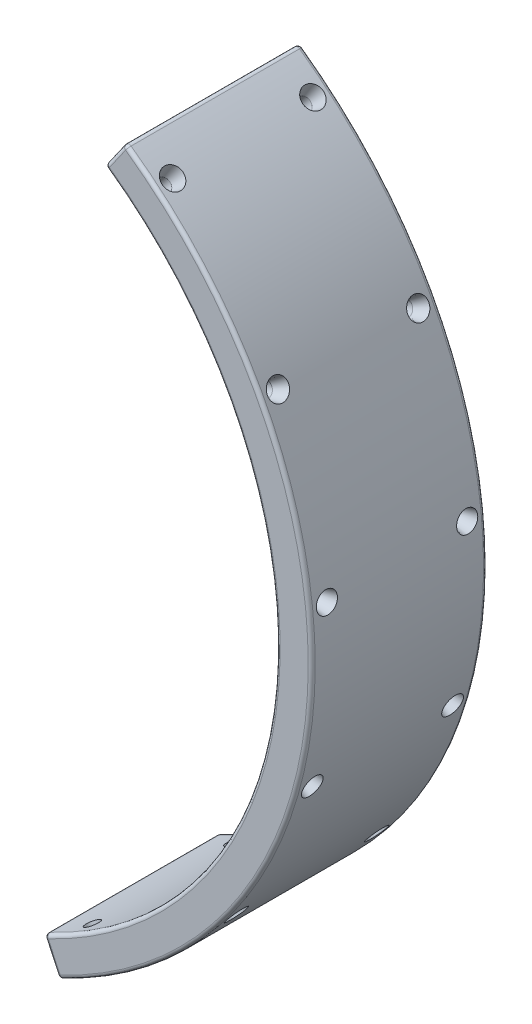
from build123d import *

# Parameters (mm, degrees)
EXTRUDE1_DEPTH             = 50
FILLET1_R                  = 2
CUT_EXTRUDE1_REACH         = 426.605
CUT_EXTRUDE1_END_RADIUS    = 230
SKETCH3_R                  = 4
CIRPATTERN1_COUNT          = 6
CIRPATTERN1_ANGLE          = 110
MIRROR1_COPY_6_REACH       = 426.605
MIRROR1_COPY_6_END_RADIUS  = 230
MIRROR1_COPY_6_SKETCH_R    = 4
MIRROR1_COPY_7_REACH       = 426.605
MIRROR1_COPY_7_END_RADIUS  = 230
MIRROR1_COPY_7_SKETCH_R    = 4
MIRROR1_COPY_8_REACH       = 426.605
MIRROR1_COPY_8_END_RADIUS  = 230
MIRROR1_COPY_8_SKETCH_R    = 4
MIRROR1_COPY_9_REACH       = 426.605
MIRROR1_COPY_9_END_RADIUS  = 230
MIRROR1_COPY_9_SKETCH_R    = 4
MIRROR1_COPY_10_REACH      = 426.605
MIRROR1_COPY_10_END_RADIUS = 230
MIRROR1_COPY_10_SKETCH_R   = 4


with BuildPart() as part:
    # Sketch1 → Extrude1 (new, symmetric)
    with BuildSketch(Plane.XY):
        with BuildLine():
            Line((143.394109088, 204.788011072), (131.922580361, 188.404970186))
            ThreePointArc((131.922580361, 188.404970186), (229.124780561, -20.045820832), (97.2022002, -208.450791018))
            Line((97.2022002, -208.450791018), (105.654565435, -226.576946759))
            ThreePointArc((105.654565435, -226.576946759), (249.048674523, -21.788935687), (143.394109088, 204.788011072))
        make_face()
    extrude(amount=EXTRUDE1_DEPTH, both=True)

    # Fillet1
    fillet1_edges = [part.edges().sort_by_distance(p)[0] for p in [
        (229.124780561, -20.045820832, 50),
        (101.428382818, -217.513868889, 50),
        (249.048674523, -21.788935687, 50),
        (101.428382818, -217.513868889, -50),
        (229.124780561, -20.045820832, -50),
        (137.658344724, 196.596490629, -50),
        (249.048674523, -21.788935687, -50),
        (137.658344724, 196.596490629, 50),
        (105.654565435, -226.576946759, 0),
        (97.2022002, -208.450791018, 0),
        (131.922580361, 188.404970186, 0),
        (143.394109088, 204.788011072, 0),
    ]]
    fillet(fillet1_edges, radius=FILLET1_R)

    # Sketch2 → Cut-Revolve2 (revolve, cut)
    with BuildSketch(Plane.XY.offset(40), mode=Mode.PRIVATE) as cut_revolve2_sk:
        Polygon((165.29316908, 187.654385122), (160.696902422, 191.51111078), (155.182894061, 184.939771506), (158.247071833, 182.368621067), align=None)
    cut_revolve2 = revolve(cut_revolve2_sk.sketch.rotate(Axis((160.696902422, 191.51111078, 40), (-0.642787609686537, -0.7660444431189801, 0)), 180), axis=Axis((160.696902422, 191.51111078, 40), (-0.642787609686537, -0.7660444431189801, 0)), mode=Mode.SUBTRACT)

    # Cut-Extrude1: up to this cylinder (the profile starts outside it)
    cut_extrude1_end = Plane(origin=(0, 0, 40), z_dir=(0, 0, -1)) * Cylinder(CUT_EXTRUDE1_END_RADIUS, 1314.21, mode=Mode.PRIVATE)
    # Sketch3 → Cut-Extrude1 (cut, up to the surface)
    with BuildSketch(Plane(origin=(155.182894061, 184.939771506, 0), x_dir=(0.7660444431189792, -0.6427876096865379, 0), z_dir=(0.6427876096865379, 0.7660444431189792, 0)), mode=Mode.PRIVATE) as cut_extrude1_sk1:
        with Locations(Location((0, -40, 0), (0, 0, 180))):
            Circle(SKETCH3_R)
    cut_extrude1_tool1 = extrude(cut_extrude1_sk1.sketch, amount=-CUT_EXTRUDE1_REACH, mode=Mode.PRIVATE) - cut_extrude1_end
    cut_extrude1 = cut_extrude1_tool1.solids().sort_by_distance((155.182894, 184.939772, 40))[0]
    add(cut_extrude1, mode=Mode.SUBTRACT)

    # CirPattern1: Cut-Revolve2, Cut-Extrude1 ×6 about axis
    cirpattern1_axis = Axis((0, 0, 48), (0, 0, -1))
    add([cut_revolve2.rotate(cirpattern1_axis, i * CIRPATTERN1_ANGLE / (CIRPATTERN1_COUNT - 1)) for i in range(1, CIRPATTERN1_COUNT)], mode=Mode.SUBTRACT)
    add([cut_extrude1.rotate(cirpattern1_axis, i * CIRPATTERN1_ANGLE / (CIRPATTERN1_COUNT - 1)) for i in range(1, CIRPATTERN1_COUNT)], mode=Mode.SUBTRACT)

    # Mirror1: Cut-Revolve2, Cut-Extrude1 across plane
    add(cut_revolve2.mirror(Plane.XY), mode=Mode.SUBTRACT)
    add(cut_extrude1.mirror(Plane.XY), mode=Mode.SUBTRACT)

    # Mirror1 copy 1 sketch → Mirror1 copy 1 (revolve, cut)
    with BuildSketch(Plane(origin=(0, 0, -40), x_dir=(0.9271838545667871, -0.37460659341591285, 0), z_dir=(0, 0, -1))):
        Polygon((165.29316908, -187.654385122), (160.696902422, -191.51111078), (155.182894061, -184.939771506), (158.247071833, -182.368621067), align=None)
    revolve(axis=Axis((220.736898215, 117.367890696, -40), (0.8829475928589261, 0.4694715627858928, 0)), mode=Mode.SUBTRACT)

    # Mirror1 copy 2 sketch → Mirror1 copy 2 (revolve, cut)
    with BuildSketch(Plane(origin=(0, 0, -40), x_dir=(0.71933980033865, -0.6946583704589985, 0), z_dir=(0, 0, -1))):
        Polygon((165.29316908, -187.654385122), (160.696902422, -191.51111078), (155.182894061, -184.939771506), (158.247071833, -182.368621067), align=None)
    revolve(axis=Axis((248.630473842, 26.132115817, -40), (0.9945218953682733, 0.10452846326765486, 0)), mode=Mode.SUBTRACT)

    # Mirror1 copy 3 sketch → Mirror1 copy 3 (revolve, cut)
    with BuildSketch(Plane(origin=(0, 0, -40), x_dir=(0.40673664307579793, -0.9135454576426019, 0), z_dir=(0, 0, -1))):
        Polygon((165.29316908, -187.654385122), (160.696902422, -191.51111078), (155.182894061, -184.939771506), (158.247071833, -182.368621067), align=None)
    revolve(axis=Axis((240.315423985, -68.909338954, -40), (0.9612616959383191, -0.2756373558169986, 0)), mode=Mode.SUBTRACT)

    # Mirror1 copy 4 sketch → Mirror1 copy 4 (revolve, cut)
    with BuildSketch(Plane(origin=(0, 0, -40), x_dir=(0.03489949670249753, -0.9993908270190959, 0), z_dir=(0, 0, -1))):
        Polygon((165.29316908, -187.654385122), (160.696902422, -191.51111078), (155.182894061, -184.939771506), (158.247071833, -182.368621067), align=None)
    revolve(axis=Axis((197.002688402, -153.915368831, -40), (0.7880107536067218, -0.6156614753256587, 0)), mode=Mode.SUBTRACT)

    # Mirror1 copy 5 sketch → Mirror1 copy 5 (revolve, cut)
    with BuildSketch(Plane(origin=(0, 0, -40), x_dir=(-0.3420201433256729, -0.9396926207859069, 0), z_dir=(0, 0, -1))):
        Polygon((165.29316908, -187.654385122), (160.696902422, -191.51111078), (155.182894061, -184.939771506), (158.247071833, -182.368621067), align=None)
    revolve(axis=Axis((125, -216.506350946, -40), (0.4999999999999989, -0.8660254037844394, 0)), mode=Mode.SUBTRACT)

    # Mirror1 copy 6: up to this cylinder (the profile starts outside it)
    mirror1_copy_6_end = Plane(origin=(0, 0, 40), z_dir=(0, 0, -1)) * Cylinder(MIRROR1_COPY_6_END_RADIUS, 1314.21, mode=Mode.PRIVATE)
    # Mirror1 copy 6 sketch → Mirror1 copy 6 (cut, up to the surface)
    with BuildSketch(Plane(origin=(213.162731669, 113.340634907, 0), x_dir=(0.4694715627858917, -0.8829475928589265, 0), z_dir=(0.8829475928589265, 0.4694715627858917, 0)), mode=Mode.PRIVATE) as mirror1_copy_6_sk1:
        with Locations((0, 40)):
            Circle(MIRROR1_COPY_6_SKETCH_R)
    mirror1_copy_6_tool1 = extrude(mirror1_copy_6_sk1.sketch, amount=-MIRROR1_COPY_6_REACH, mode=Mode.PRIVATE) - mirror1_copy_6_end
    add(mirror1_copy_6_tool1.solids().sort_by_distance((155.182894, 184.939772, 40))[0], mode=Mode.SUBTRACT)

    # Mirror1 copy 7: up to this cylinder (the profile starts outside it)
    mirror1_copy_7_end = Plane(origin=(0, 0, 40), z_dir=(0, 0, -1)) * Cylinder(MIRROR1_COPY_7_END_RADIUS, 1314.21, mode=Mode.PRIVATE)
    # Mirror1 copy 7 sketch → Mirror1 copy 7 (cut, up to the surface)
    with BuildSketch(Plane(origin=(240.099192337, 25.235441998, 0), x_dir=(0.10452846326765369, -0.9945218953682733, 0), z_dir=(0.9945218953682733, 0.10452846326765369, 0)), mode=Mode.PRIVATE) as mirror1_copy_7_sk1:
        with Locations((0, 40)):
            Circle(MIRROR1_COPY_7_SKETCH_R)
    mirror1_copy_7_tool1 = extrude(mirror1_copy_7_sk1.sketch, amount=-MIRROR1_COPY_7_REACH, mode=Mode.PRIVATE) - mirror1_copy_7_end
    add(mirror1_copy_7_tool1.solids().sort_by_distance((155.182894, 184.939772, 40))[0], mode=Mode.SUBTRACT)

    # Mirror1 copy 8: up to this cylinder (the profile starts outside it)
    mirror1_copy_8_end = Plane(origin=(0, 0, 40), z_dir=(0, 0, -1)) * Cylinder(MIRROR1_COPY_8_END_RADIUS, 1314.21, mode=Mode.PRIVATE)
    # Mirror1 copy 8 sketch → Mirror1 copy 8 (cut, up to the surface)
    with BuildSketch(Plane(origin=(232.06945759, -66.544846139, 0), x_dir=(-0.2756373558169998, -0.9612616959383187, 0), z_dir=(0.9612616959383187, -0.2756373558169998, 0)), mode=Mode.PRIVATE) as mirror1_copy_8_sk1:
        with Locations((0, 40)):
            Circle(MIRROR1_COPY_8_SKETCH_R)
    mirror1_copy_8_tool1 = extrude(mirror1_copy_8_sk1.sketch, amount=-MIRROR1_COPY_8_REACH, mode=Mode.PRIVATE) - mirror1_copy_8_end
    add(mirror1_copy_8_tool1.solids().sort_by_distance((155.182894, 184.939772, 40))[0], mode=Mode.SUBTRACT)

    # Mirror1 copy 9: up to this cylinder (the profile starts outside it)
    mirror1_copy_9_end = Plane(origin=(0, 0, 40), z_dir=(0, 0, -1)) * Cylinder(MIRROR1_COPY_9_END_RADIUS, 1314.21, mode=Mode.PRIVATE)
    # Mirror1 copy 9 sketch → Mirror1 copy 9 (cut, up to the surface)
    with BuildSketch(Plane(origin=(190.242916094, -148.634055889, 0), x_dir=(-0.6156614753256596, -0.7880107536067209, 0), z_dir=(0.7880107536067209, -0.6156614753256596, 0)), mode=Mode.PRIVATE) as mirror1_copy_9_sk1:
        with Locations((0, 40)):
            Circle(MIRROR1_COPY_9_SKETCH_R)
    mirror1_copy_9_tool1 = extrude(mirror1_copy_9_sk1.sketch, amount=-MIRROR1_COPY_9_REACH, mode=Mode.PRIVATE) - mirror1_copy_9_end
    add(mirror1_copy_9_tool1.solids().sort_by_distance((155.182894, 184.939772, 40))[0], mode=Mode.SUBTRACT)

    # Mirror1 copy 10: up to this cylinder (the profile starts outside it)
    mirror1_copy_10_end = Plane(origin=(0, 0, 40), z_dir=(0, 0, -1)) * Cylinder(MIRROR1_COPY_10_END_RADIUS, 1314.21, mode=Mode.PRIVATE)
    # Mirror1 copy 10 sketch → Mirror1 copy 10 (cut, up to the surface)
    with BuildSketch(Plane(origin=(120.710862906, -209.077347578, 0), x_dir=(-0.8660254037844399, -0.49999999999999784, 0), z_dir=(0.49999999999999784, -0.8660254037844399, 0)), mode=Mode.PRIVATE) as mirror1_copy_10_sk1:
        with Locations((0, 40)):
            Circle(MIRROR1_COPY_10_SKETCH_R)
    mirror1_copy_10_tool1 = extrude(mirror1_copy_10_sk1.sketch, amount=-MIRROR1_COPY_10_REACH, mode=Mode.PRIVATE) - mirror1_copy_10_end
    add(mirror1_copy_10_tool1.solids().sort_by_distance((155.182894, 184.939772, 40))[0], mode=Mode.SUBTRACT)


solid = part.part
